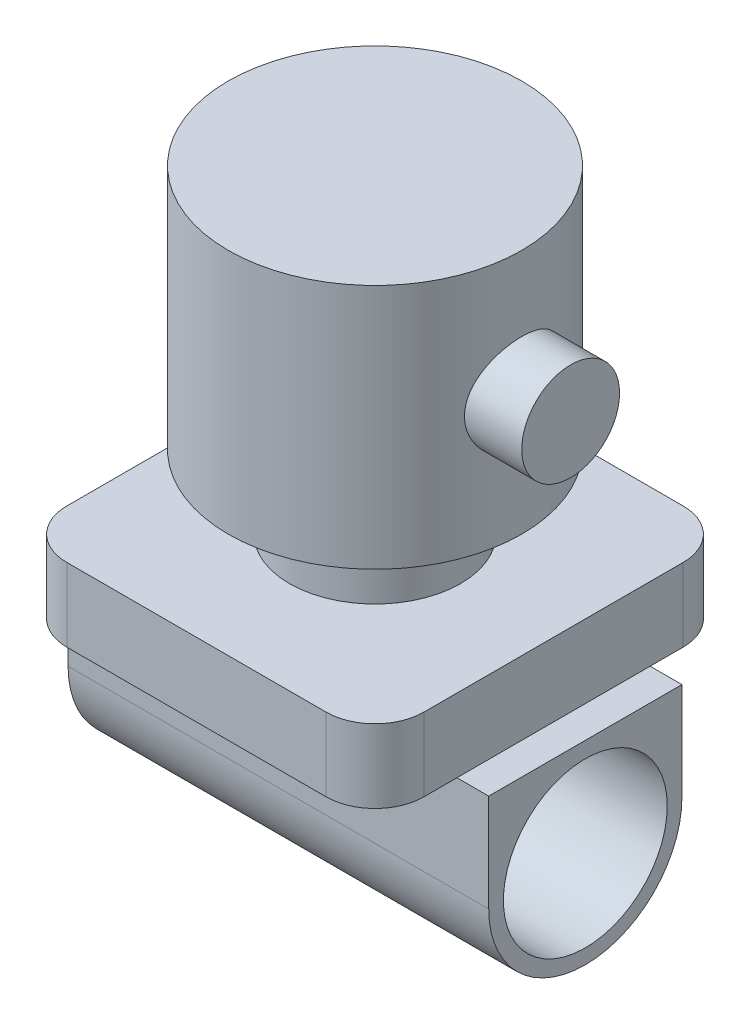
SolidWorks part; units mm, degrees
material "黄铜"
ref_plane "前视基准面" through (0, 0, 0) normal (0, 0, 1) x (1, 0, 0)
ref_plane "上视基准面" through (0, 0, 0) normal (0, 1, 0) x (1, 0, 0)
ref_plane "右视基准面" through (0, 0, 0) normal (1, 0, 0) x (0, 0, -1)
sketch "草图1" plane through (0, 0, 0) normal (1, 0, 0) x (0, 0, -1)
  circle A0 centre (0, 0) radius 16.75
  dimension "D1" = 33.5
extrude "拉伸-薄壁1" add sketch "草图1" along normal mid plane 86 thin
ref_plane "基准面1" through (0, 20, 0) normal (0, 1, 0) x (1, 0, 0)
sketch "草图3" plane through (0, 20, 0) normal (0, 1, 0) x (1, 0, 0)
  line L1 (-26.5, 36.5) -> (26.5, 36.5)
  line L2 (-36.5, 26.5) -> (-36.5, -26.5)
  line L3 (-26.5, -36.5) -> (26.5, -36.5)
  line L4 (36.5, 26.5) -> (36.5, -26.5)
  arc A0 (-26.5, -36.5) -> (-36.5, -26.5) centre (-26.5, -26.5) cw
  arc A1 (36.5, -26.5) -> (26.5, -36.5) centre (26.5, -26.5) cw
  arc A2 (36.5, 26.5) -> (26.5, 36.5) centre (26.5, 26.5) ccw
  arc A3 (-26.5, 36.5) -> (-36.5, 26.5) centre (-26.5, 26.5) ccw
  point P7 (-36.5, -36.5)
  point P12 (36.5, 36.5)
  point P15 (-36.5, 36.5)
  dimension "D5" = 10
  dimension "D1" = 73
  dimension "D2" = 73
  dimension "D3" = 36.5
  dimension "D4" = 36.5
extrude "凸台-拉伸1" add sketch "草图3" along normal blind 15 separate body
sketch "草图4" plane through (0, 35, 0) normal (0, 1, 0) x (1, 0, 0)
  circle A0 centre (0, 0) radius 17.5
  dimension "D1" = 35
extrude "凸台-拉伸2" add sketch "草图4" along normal blind 15
sketch "草图5" plane through (0, 50, 0) normal (0, 1, 0) x (1, 0, 0)
  circle A0 centre (0, 0) radius 30
  dimension "D1" = 60
extrude "凸台-拉伸3" add sketch "草图5" along normal blind 50.25
sketch "草图6" plane through (43, 0, 0) normal (1, 0, 0) x (0, 0, -1)
  line L0 (40.15, 20) -> (-40.15, 20) construction
  line L2 (-19.75, 0) -> (-19.75, 20)
  line L3 (-19.75, 20) -> (19.75, 20)
  line L4 (19.75, 0) -> (19.75, 20)
  arc A0 (19.75, 0) -> (-19.75, 0) centre (0, 0) ccw
extrude "凸台-拉伸4" add sketch "草图6" against normal up to surface (86 mm away)
ref_plane "基准面2" through (40, 0, 0) normal (1, 0, 0) x (0, 0, -1)
sketch "草图7" plane through (40, 0, 0) normal (1, 0, 0) x (0, 0, -1)
  line L0 (-30, 50) -> (30, 50) construction
  circle A0 centre (0, 75) radius 10
  dimension "D1" = 20
  dimension "D2" = 25
extrude "凸台-拉伸5" add sketch "草图7" against normal up to surface (11.7157 mm away)
